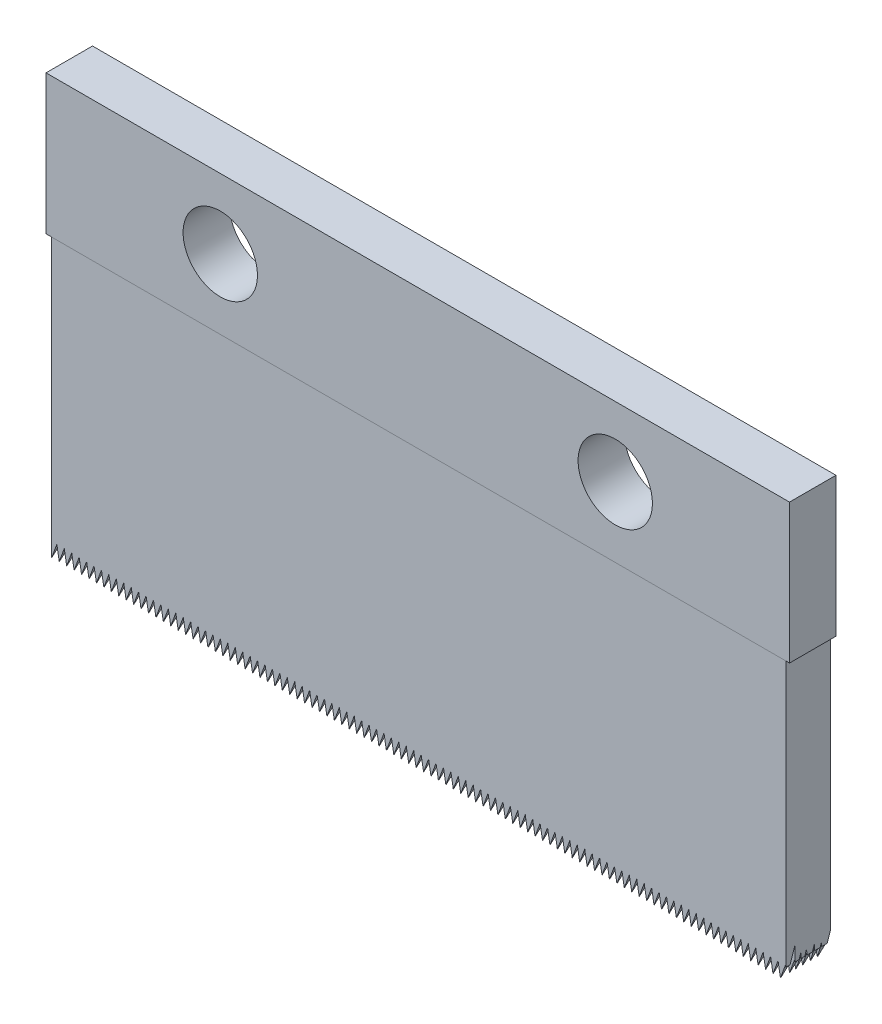
from build123d import *

# Parameters (mm, degrees)
SKETCH_1_W             = 80
SKETCH_1_H             = 15
SKETCH_1_R             = 4
EXTRUDE_1_DEPTH        = 5
SKETCH_2_W             = 79
SKETCH_2_H             = 4.8
EXTRUDE_2_DEPTH        = 30
CUT_EXTRUDE_1_DEPTH    = 90
CUT_EXTRUDE_2_DEPTH    = 90
PATTERN_LINEAR_1_COUNT = 102
PATTERN_LINEAR_1_PITCH = 0.8


with BuildPart() as part:
    # 草图1 → 凸台-拉伸1 (new body)
    with BuildSketch(Plane.XY):
        Rectangle(SKETCH_1_W, SKETCH_1_H)
        with Locations((-21.25, 0)):
            Circle(SKETCH_1_R, mode=Mode.SUBTRACT)
        with Locations((21.25, 0)):
            Circle(SKETCH_1_R, mode=Mode.SUBTRACT)
    extrude(amount=EXTRUDE_1_DEPTH)

    # 草图2 → 凸台-拉伸2 (add)
    with BuildSketch(Plane.XZ.offset(7.5)):
        with Locations((0, 2.5)):
            Rectangle(SKETCH_2_W, SKETCH_2_H)
    extrude(amount=EXTRUDE_2_DEPTH)

    # 草图3 → 切除-拉伸1 (cut)
    with BuildSketch(Plane(origin=(39.5, 0, 0), x_dir=(0, 0, -1), z_dir=(1, 0, 0))):
        Polygon((-4.9, -37.5), (-3.919892463, -34.6116568), (-3.919892463, -37.5), (-3.259066216, -35.552567781), (-3.259066216, -37.5), (-2.668438693, -35.529929653), (-2.5, -37.5), (-1.833427845, -35.555241046), (-1.667153246, -37.5), (-1.064855763, -35.742765745), (-0.914614305, -37.5), (-0.1, -35.123320368), (4.756459171, -37.5), (-2.083576623, -39.323662605), (-4.9, -38.835895592), align=None)
    extrude(amount=-CUT_EXTRUDE_1_DEPTH, mode=Mode.SUBTRACT)

    # 草图4 → 切除-拉伸2 (cut)
    with BuildSketch(Plane.XY.offset(4.9)):
        Polygon((-39.5, -37.5), (-38.935119687, -35.948004096), (-38.666110535, -37.5), (-38.666110535, -38.237675699), align=None)
    cut_extrude_2 = extrude(amount=-CUT_EXTRUDE_2_DEPTH, mode=Mode.SUBTRACT)

    # 阵列(线性)1: 切除-拉伸2 ×102
    with Locations(*[(i * PATTERN_LINEAR_1_PITCH, 0, 0) for i in range(1, PATTERN_LINEAR_1_COUNT)]):
        add(cut_extrude_2, mode=Mode.SUBTRACT)


solid = part.part
